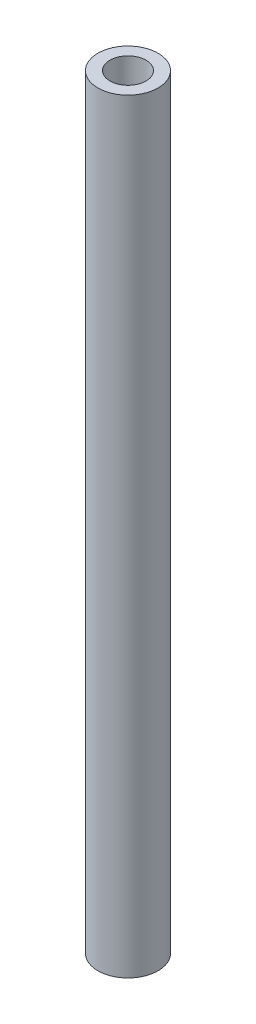
SolidWorks part; units mm, degrees
ref_plane "Front Plane" through (0, 0, 0) normal (0, 0, 1) x (1, 0, 0)
ref_plane "Top Plane" through (0, 0, 0) normal (0, 1, 0) x (1, 0, 0)
ref_plane "Right Plane" through (0, 0, 0) normal (1, 0, 0) x (0, 0, -1)
sketch "Sketch1" plane through (0, 0, 0) normal (0, 1, 0) x (1, 0, 0)
  circle A0 centre (0, 0) radius 2.5
  circle A1 centre (0, 0) radius 1.5
  dimension "D1" = 5
  dimension "D2" = 3
extrude "Boss-Extrude1" add sketch "Sketch1" along normal blind 63.5
cosmetic thread "Cosmetic Thread1" parameters "D1"=5, "D2"=4
sketch "Sketch2" plane through (0, 0, 0) normal (0, -1, 0) x (1, 0, 0)
  circle A0 centre (0, 0) radius 1.5 construction
  circle A1 centre (0, 0) radius 1.5
  circle A2 centre (0, 0) radius 0.5
  dimension "D1" = 1
extrude "Boss-Extrude2" add sketch "Sketch2" against normal blind 2
